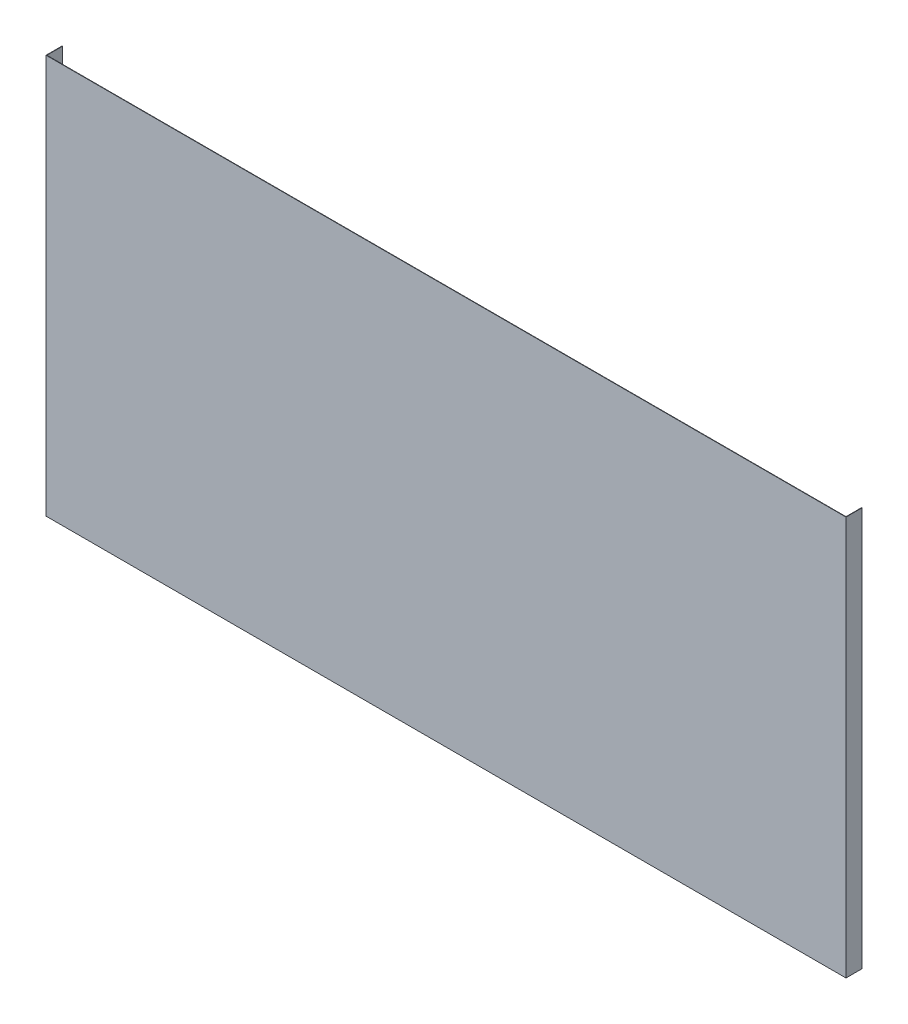
SolidWorks part; units mm, degrees
ref_plane "前视基准面" through (0, 0, 0) normal (0, 0, 1) x (1, 0, 0)
ref_plane "上视基准面" through (0, 0, 0) normal (0, 1, 0) x (1, 0, 0)
ref_plane "右视基准面" through (0, 0, 0) normal (1, 0, 0) x (0, 0, -1)
sketch "草图1" plane through (0, 0, 0) normal (0, 0, 1) x (1, 0, 0)
  line L1 (-2002, 1000) -> (2002, 1000)
  line L2 (-2002, 1000) -> (-2002, -1000)
  line L3 (-2002, -1000) -> (2002, -1000)
  line L4 (2002, 1000) -> (2002, -1000)
  line L5 (-2002, 1000) -> (2002, -1000) construction
  line L6 (-2002, -1000) -> (2002, 1000) construction
  point P0 (0, 0)
  dimension "D1" = 4004
  dimension "D2" = 2000
extrude "凸台-拉伸1" add sketch "草图1" along normal blind 2
sketch "草图2" plane through (-2002, 0, 0) normal (-1, 0, 0) x (0, 0, 1)
  line L1 (2, 1000) -> (-78, 1000)
  line L2 (2, 1000) -> (2, -1000)
  line L3 (2, -1000) -> (-78, -1000)
  line L4 (-78, 1000) -> (-78, -1000)
  dimension "D1" = 80
extrude "凸台-拉伸2" add sketch "草图2" along normal blind 2
sketch "草图3" plane through (2002, 0, 0) normal (1, 0, 0) x (0, 0, -1)
  line L4 (78, 1000) -> (-2, 1000)
  line L5 (78, -1000) -> (78, 1000)
  line L6 (-2, -1000) -> (78, -1000)
  line L7 (-2, 1000) -> (-2, -1000)
  line L8 (78, 1000) -> (-2, 1000)
  line L9 (78, -1000) -> (78, 1000)
  line L10 (-2, -1000) -> (78, -1000)
  line L11 (-2, 1000) -> (-2, -1000)
  dimension "D1" = 0
extrude "凸台-拉伸3" add sketch "草图3" along normal blind 2
